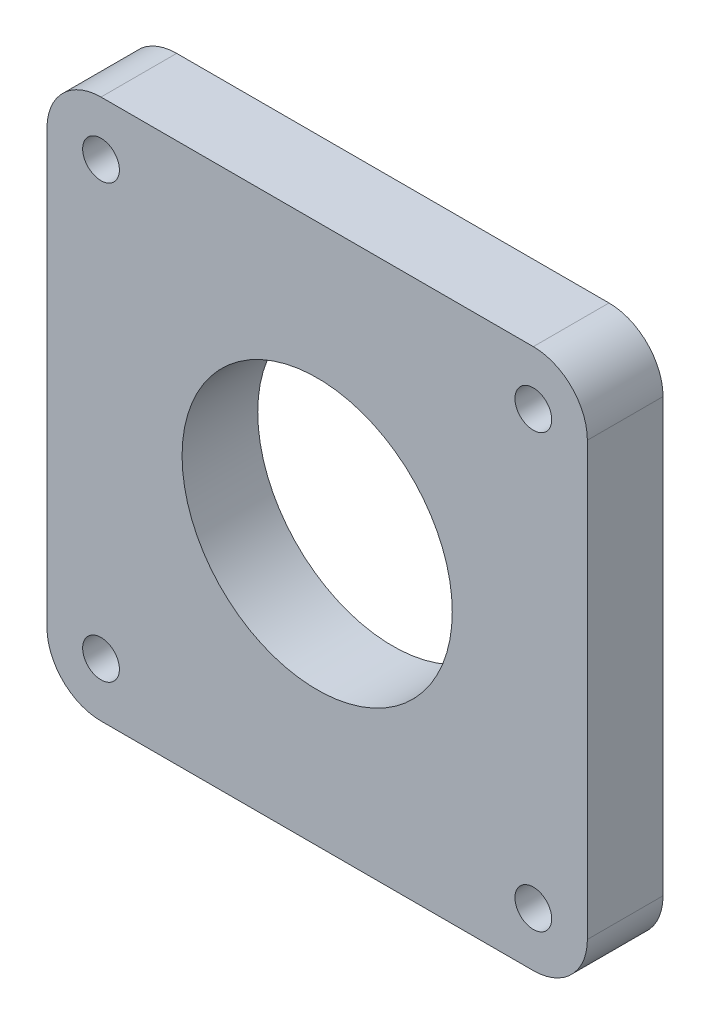
SolidWorks part; units mm, degrees
ref_plane "Front" through (0, 0, 0) normal (0, 0, 1) x (1, 0, 0)
ref_plane "Top" through (0, 0, 0) normal (0, 1, 0) x (1, 0, 0)
ref_plane "Right" through (0, 0, 0) normal (1, 0, 0) x (0, 0, -1)
sketch "Sketch1" plane through (0, 0, 0) normal (0, 0, 1) x (1, 0, 0)
  line L1 (0, 0) -> (100, 0)
  line L2 (0, 0) -> (0, -100)
  line L3 (0, -100) -> (100, -100)
  line L4 (100, 0) -> (100, -100)
  dimension "D1" = 100
  dimension "D2" = 100
extrude "Boss-Extrude1" add sketch "Sketch1" along normal blind 14
sketch "Sketch2" plane through (0, 0, 14) normal (0, 0, 1) x (1, 0, 0)
  line L0 (0, -50) -> (50, -50) construction
  line L1 (0, 0) -> (0, -100) construction
  line L2 (50, 0) -> (50, -50) construction
  line L3 (100, 0) -> (0, 0) construction
  circle A0 centre (50, -50) radius 25
  dimension "D1" = 50
extrude "Cut-Extrude1" cut sketch "Sketch2" against normal through all
hole_wizard "M8 Tapped Hole1" positions "Sketch3" profile "Sketch4" tap size "M8" standard "GB" end condition through all
sketch "Sketch3" plane through (0, 0, 14) normal (0, 0, 1) x (1, 0, 0)
  line L1 (50, 0) -> (50, -100) construction
  line L2 (100, 0) -> (0, 0) construction
  line L3 (0, -100) -> (100, -100) construction
  line L5 (50, -50) -> (100, -50) construction
  line L6 (100, -100) -> (100, 0) construction
  point P0 (10, -10)
  point P2 (90, -10)
  point P4 (10, -90)
  point P6 (90, -90)
  dimension "D1" = 80
  dimension "D2" = 80
sketch "Sketch4" plane through (10, -10, 14) normal (1, 0, 0) x (0, -1, 0)
  line L0 (0, 0) -> (0, 14)
  line L1 (0, 14) -> (3.4, 14)
  line L2 (3.4, 14) -> (3.4, 0)
  line L5 (3.4, 0) -> (0, 0)
  line L11 (0, -6.35) -> (0, 107.95) construction
  dimension "通孔螺纹孔钻头直径" = 6.8
  dimension "通孔螺纹孔钻头深度" = 14
cosmetic thread "Hole Thread Line1" parameters "D2"=8
cosmetic thread "Hole Thread Line2" parameters "D2"=8
cosmetic thread "Hole Thread Line3" parameters "D2"=8
cosmetic thread "Hole Thread Line4" parameters "D2"=8
sketch "Sketch5" plane through (0, 0, 14) normal (0, 0, 1) x (1, 0, 0)
  circle A0 centre (50, -50) radius 30
  dimension "D1" = 60
extrude "Boss-Extrude2" [suppressed] add sketch "Sketch5" along normal blind 316
fillet "Fillet1" radius 10 4 edges at (0, -100, 7) (100, -100, 7) (100, 0, 7) (0, 0, 7)
